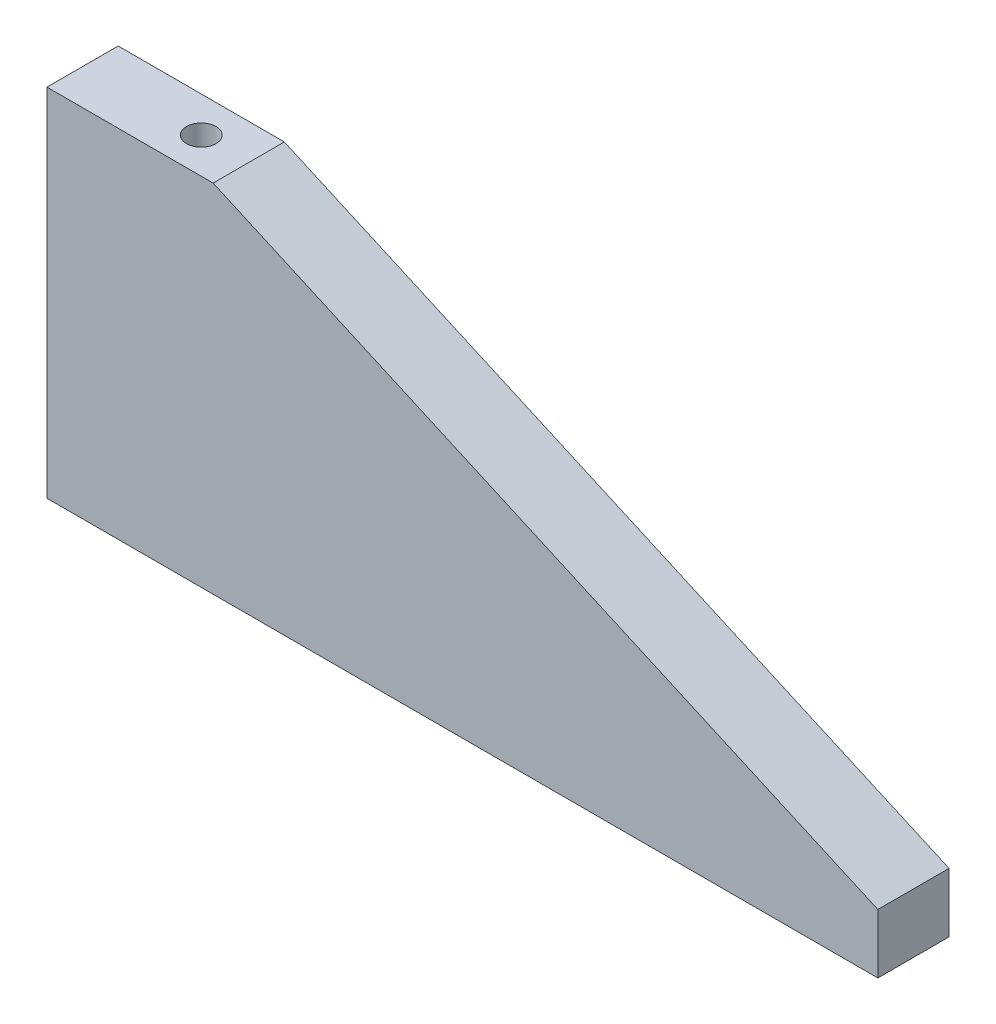
SolidWorks part; units mm, degrees
ref_plane "前视" through (0, 0, 0) normal (0, 0, 1) x (1, 0, 0)
ref_plane "上视" through (0, 0, 0) normal (0, 1, 0) x (1, 0, 0)
ref_plane "右视" through (0, 0, 0) normal (1, 0, 0) x (0, 0, -1)
sketch "草图1" plane through (0, 0, 0) normal (0, 0, 1) x (1, 0, 0)
  line L0 (0, 0) -> (0, -60)
  line L1 (0, -60) -> (140, -60)
  line L2 (140, -60) -> (140, -50)
  line L3 (140, -50) -> (28, 0)
  line L4 (28, 0) -> (0, 0)
  dimension "D1" = 60
  dimension "D2" = 28
  dimension "D3" = 140
  dimension "D4" = 10
extrude "凸台-拉伸1" add sketch "草图1" along normal blind 12
hole_wizard "M6 螺纹孔1" positions "草图3" profile "草图2" tap size "M6" standard "ISO"
sketch "草图3" plane through (0, 0, 0) normal (-1, 0, 0) x (0, 0, 1)
  line L0 (6, 0) -> (6, -15) construction
  line L1 (12, 0) -> (0, 0) construction
  line L2 (6, -15) -> (6, -45) construction
  point P0 (6, -15)
  point P2 (6, -45)
  dimension "D1" = 15
  dimension "D2" = 30
sketch "草图2" plane through (0, -15, 6) normal (0, 1, 0) x (0, 0, 1)
  line L0 (0, 0) -> (0, 16.5022)
  line L1 (0, 16.5022) -> (2.5, 15)
  line L2 (2.5, 15) -> (2.5, 0)
  line L5 (2.5, 0) -> (0, 0)
  line L10 (0, 16.5022) -> (-2.5, 15) construction
  line L11 (0, -6.35) -> (0, 107.95) construction
  dimension "螺纹孔钻头直径" = 5
  dimension "螺纹孔钻头深度" = 15
  dimension "导头角度" = 118
cosmetic thread "孔螺蚊线1"
cosmetic thread "孔螺蚊线2"
hole_wizard "M6 螺纹孔2" positions "草图5" profile "草图4" tap size "M6" standard "ISO"
sketch "草图5" plane through (0, -60, 0) normal (0, -1, 0) x (-1, 0, 0)
  line L0 (-140, -6) -> (-120, -6) construction
  line L1 (-140, -12) -> (-140, 0) construction
  line L2 (-120, -6) -> (-20, -6) construction
  line L3 (0, -12) -> (0, 0) construction
  point P0 (-120, -6)
  point P2 (-20, -6)
  dimension "D1" = 20
  dimension "D2" = 100
sketch "草图4" plane through (120, -60, 6) normal (1, 0, 0) x (0, 0, -1)
  line L0 (0, 0) -> (0, 16.5022)
  line L1 (0, 16.5022) -> (2.5, 15)
  line L2 (2.5, 15) -> (2.5, 0)
  line L5 (2.5, 0) -> (0, 0)
  line L10 (0, 16.5022) -> (-2.5, 15) construction
  line L11 (0, -6.35) -> (0, 107.95) construction
  dimension "螺纹孔钻头直径" = 5
  dimension "螺纹孔钻头深度" = 15
  dimension "导头角度" = 118
cosmetic thread "孔螺蚊线3"
cosmetic thread "孔螺蚊线4"
hole_wizard "M6 螺纹孔3" positions "草图7" profile "草图6" tap size "M6" standard "ISO"
sketch "草图7" plane through (0, 0, 0) normal (0, 1, 0) x (1, 0, 0)
  line L0 (0, -6) -> (20, -6) construction
  line L1 (0, -12) -> (0, 0) construction
  point P0 (20, -6)
  dimension "D1" = 20
sketch "草图6" plane through (20, 0, 6) normal (1, 0, 0) x (0, 0, 1)
  line L0 (0, 0) -> (0, 16.5022)
  line L1 (0, 16.5022) -> (2.5, 15)
  line L2 (2.5, 15) -> (2.5, 0)
  line L5 (2.5, 0) -> (0, 0)
  line L10 (0, 16.5022) -> (-2.5, 15) construction
  line L11 (0, -6.35) -> (0, 107.95) construction
  dimension "螺纹孔钻头直径" = 5
  dimension "螺纹孔钻头深度" = 15
  dimension "导头角度" = 118
cosmetic thread "孔螺蚊线5"
